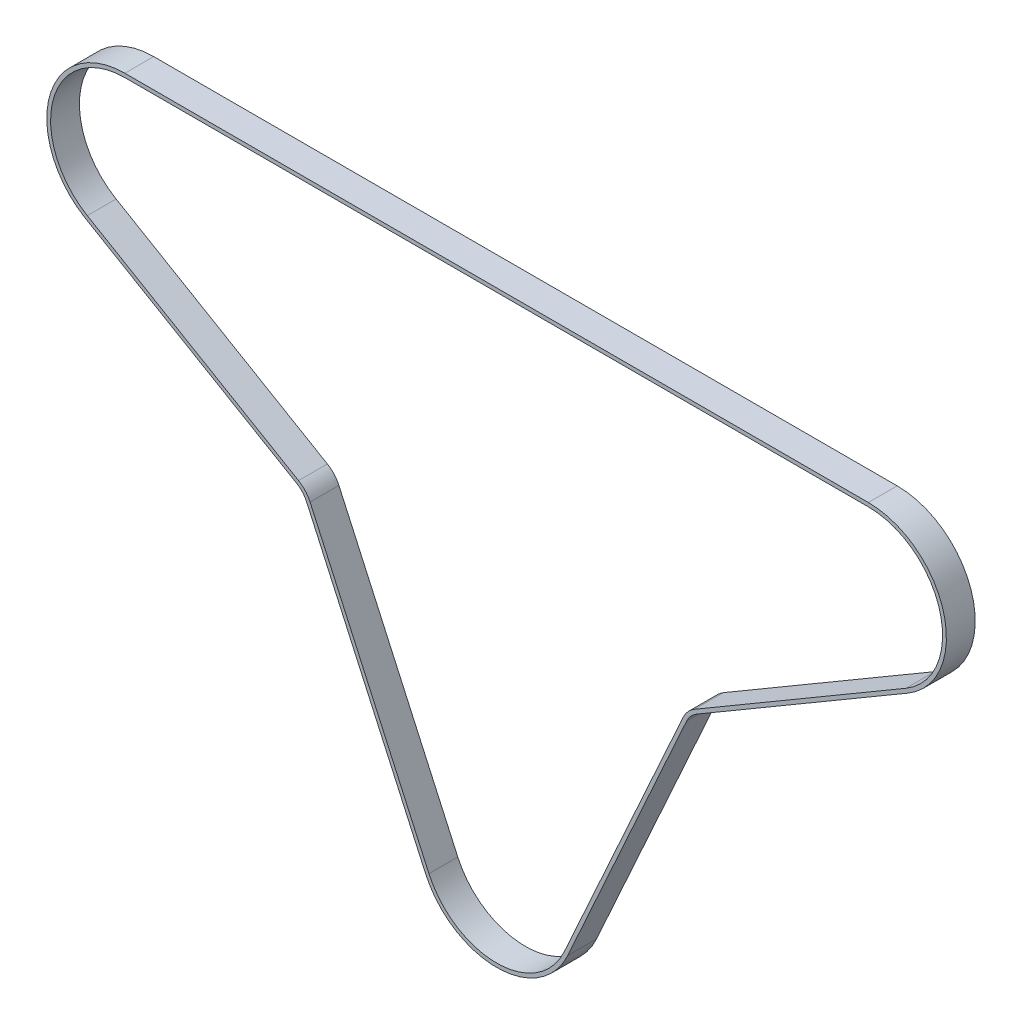
from build123d import *

# Parameters (mm, degrees)
EXTRUDE_1_DEPTH = 19


with BuildPart() as part:
    # 草图2 → 拉伸-薄壁1 (new, symmetric)
    with BuildSketch(Plane.XY):
        with BuildLine():
            Line((250.396106976, 303.41117138), (93.71226198, -42.453604657))
            ThreePointArc((93.71226198, -42.453604657), (0, -102.880025838), (-93.71226198, -42.453604657))
            Line((-93.71226198, -42.453604657), (-250.396106976, 303.41117138))
            ThreePointArc((-250.396106976, 303.41117138), (-255.847210975, 311.746098094), (-263.566345627, 318.03899078))
            Line((-263.566345627, 318.03899078), (-542.021364981, 481.241496264))
            ThreePointArc((-542.021364981, 481.241496264), (-589.286880464, 596.951990053), (-490, 672.88))
            Line((-490, 672.88), (490, 672.88))
            ThreePointArc((490, 672.88), (589.286880464, 596.951990053), (542.021364981, 481.241496264))
            Line((542.021364981, 481.241496264), (263.566345627, 318.03899078))
            ThreePointArc((263.566345627, 318.03899078), (255.847210975, 311.746098094), (250.396106976, 303.41117138))
        make_face()
        with BuildLine():
            Line((245.841661895, 305.474428516), (89.1578169, -40.390347521))
            ThreePointArc((89.1578169, -40.390347521), (0, -97.880025838), (-89.1578169, -40.390347521))
            Line((-89.1578169, -40.390347521), (-245.841661895, 305.474428516))
            ThreePointArc((-245.841661895, 305.474428516), (-252.131397279, 315.091651647), (-261.038091108, 322.352681669))
            Line((-261.038091108, 322.352681669), (-539.493110463, 485.555187153))
            ThreePointArc((-539.493110463, 485.555187153), (-584.461507191, 595.642114953), (-490, 667.88))
            Line((-490, 667.88), (490, 667.88))
            ThreePointArc((490, 667.88), (584.461507191, 595.642114953), (539.493110463, 485.555187153))
            Line((539.493110463, 485.555187153), (261.038091108, 322.352681669))
            ThreePointArc((261.038091108, 322.352681669), (252.131397279, 315.091651647), (245.841661895, 305.474428516))
        make_face(mode=Mode.SUBTRACT)
    extrude(amount=EXTRUDE_1_DEPTH, both=True)


solid = part.part
